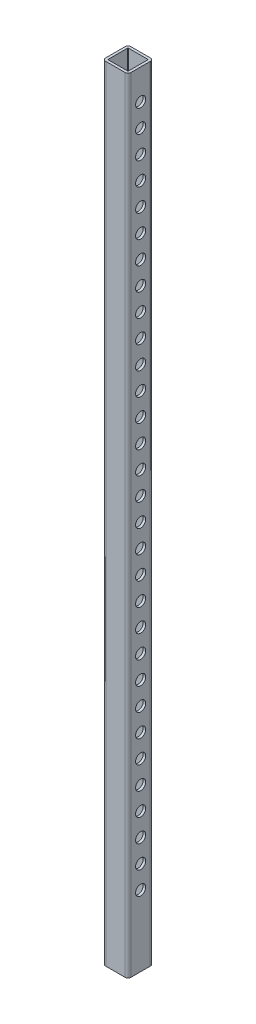
SolidWorks part; units mm, degrees
ref_plane "Front" through (0, 0, 0) normal (0, 0, 1) x (1, 0, 0)
ref_plane "Top" through (0, 0, 0) normal (0, 1, 0) x (1, 0, 0)
ref_plane "Right" through (0, 0, 0) normal (1, 0, 0) x (0, 0, -1)
sketch "草图1" plane through (0, 0, 0) normal (0, 1, 0) x (1, 0, 0)
  line L0 (-19, -7.2781) -> (19, -7.2781)
  line L1 (-19, -12.2781) -> (19, -12.2781)
  line L2 (-25, -6.2781) -> (-25, 31.7219)
  line L3 (-19, 37.7219) -> (19, 37.7219)
  line L4 (25, -6.2781) -> (25, 31.7219)
  line L5 (20, -6.2781) -> (20, 31.7219)
  line L6 (-19, 32.7219) -> (19, 32.7219)
  line L11 (-20, -6.2781) -> (-20, 31.7219)
  arc A0 (-19, -12.2781) -> (-25, -6.2781) centre (-19, -6.2781) cw
  arc A1 (19, -12.2781) -> (25, -6.2781) centre (19, -6.2781) ccw
  arc A2 (19, 37.7219) -> (25, 31.7219) centre (19, 31.7219) cw
  arc A3 (-25, 31.7219) -> (-19, 37.7219) centre (-19, 31.7219) cw
  arc A4 (19, -7.2781) -> (20, -6.2781) centre (19, -6.2781) ccw
  arc A5 (19, 32.7219) -> (20, 31.7219) centre (19, 31.7219) cw
  arc A6 (-20, 31.7219) -> (-19, 32.7219) centre (-19, 31.7219) cw
  arc A7 (-19, -7.2781) -> (-20, -6.2781) centre (-19, -6.2781) cw
  point P9 (25, -12.2781)
  point P12 (25, 37.7219)
  point P15 (-25, 37.7219)
  dimension "D3" = 6
  dimension "D1" = 50
  dimension "D2" = 50
  dimension "D4" = 5
extrude "凸台-拉伸1" add sketch "草图1" along normal blind 1550
sketch "草图2" plane through (25, 0, 0) normal (1, 0, 0) x (0, 0, -1)
  line L0 (37.7219, 1550) -> (37.7219, 0) construction
  line L1 (-6.2781, 1550) -> (31.7219, 1550) construction
  circle A0 centre (12.7219, 1527.5) radius 12
  circle A1 centre (12.7219, 1482.5) radius 12
  circle A2 centre (12.7219, 1437.5) radius 12
  circle A3 centre (12.7219, 1392.5) radius 12
  circle A4 centre (12.7219, 1347.5) radius 12
  circle A5 centre (12.7219, 1302.5) radius 12
  circle A6 centre (12.7219, 1257.5) radius 12
  circle A7 centre (12.7219, 1212.5) radius 12
  circle A8 centre (12.7219, 1167.5) radius 12
  circle A9 centre (12.7219, 1122.5) radius 12
  circle A10 centre (12.7219, 1077.5) radius 12
  circle A11 centre (12.7219, 1032.5) radius 12
  circle A12 centre (12.7219, 987.5) radius 12
  circle A13 centre (12.7219, 942.5) radius 12
  circle A14 centre (12.7219, 897.5) radius 12
  dimension "D1" = 24
  dimension "D2" = 25
  dimension "D3" = 22.5
  dimension "D4" = 15
extrude "切除-拉伸1" cut sketch "草图2" against normal blind 10
sketch "草图3" plane through (25, 0, 0) normal (1, 0, 0) x (0, 0, -1)
  circle A0 centre (12.7219, 897.5) radius 16.0651
  circle A1 centre (12.7219, 1527.5) radius 15.4417
extrude "凸台-拉伸2" add sketch "草图3" against normal up to surface (5 mm away) up to face at (20, 1527.5, -0.7219)
sketch "草图4" plane through (25, 0, 0) normal (1, 0, 0) x (0, 0, -1)
  line L0 (-6.2781, 1550) -> (-6.2781, 0) construction
  line L1 (-6.2781, 881.4016) -> (31.7219, 881.4016)
  line L2 (-6.2781, 881.4016) -> (-6.2781, 1511.8926)
  line L3 (-6.2781, 1511.8926) -> (31.7219, 1511.8926)
  line L4 (31.7219, 881.4016) -> (31.7219, 1511.8926)
  line L5 (31.7219, 1550) -> (31.7219, 0) construction
extrude "凸台-拉伸3" add sketch "草图4" against normal up to surface (5 mm away) up to face at (20, 1482.5, -0.7219)
sketch "草图5" plane through (25, 0, 0) normal (1, 0, 0) x (0, 0, -1)
  line L0 (-6.2781, 1550) -> (31.7219, 1550) construction
  line L1 (37.7219, 1550) -> (37.7219, 0) construction
  circle A0 centre (12.7219, 1490) radius 10
  circle A1 centre (12.7219, 1445) radius 10
  circle A2 centre (12.7219, 1400) radius 10
  circle A3 centre (12.7219, 1355) radius 10
  circle A4 centre (12.7219, 1310) radius 10
  circle A5 centre (12.7219, 1265) radius 10
  circle A6 centre (12.7219, 1220) radius 10
  circle A7 centre (12.7219, 1175) radius 10
  circle A8 centre (12.7219, 1130) radius 10
  circle A9 centre (12.7219, 1085) radius 10
  circle A10 centre (12.7219, 1040) radius 10
  circle A11 centre (12.7219, 995) radius 10
  circle A12 centre (12.7219, 950) radius 10
  circle A13 centre (12.7219, 905) radius 10
  circle A14 centre (12.7219, 860) radius 10
  circle A15 centre (12.7219, 815) radius 10
  circle A16 centre (12.7219, 770) radius 10
  circle A17 centre (12.7219, 725) radius 10
  circle A18 centre (12.7219, 680) radius 10
  circle A19 centre (12.7219, 635) radius 10
  circle A20 centre (12.7219, 590) radius 10
  circle A21 centre (12.7219, 545) radius 10
  circle A22 centre (12.7219, 500) radius 10
  circle A23 centre (12.7219, 455) radius 10
  circle A24 centre (12.7219, 410) radius 10
  circle A25 centre (12.7219, 365) radius 10
  circle A26 centre (12.7219, 320) radius 10
  circle A27 centre (12.7219, 275) radius 10
  circle A28 centre (12.7219, 230) radius 10
  circle A29 centre (12.7219, 185) radius 10
  circle A30 centre (12.7219, 140) radius 10
  dimension "D2" = 25
  dimension "D3" = 20
  dimension "D1" = 60
  dimension "D4" = 31
extrude "切除-拉伸2" cut sketch "草图5" against normal blind 10
